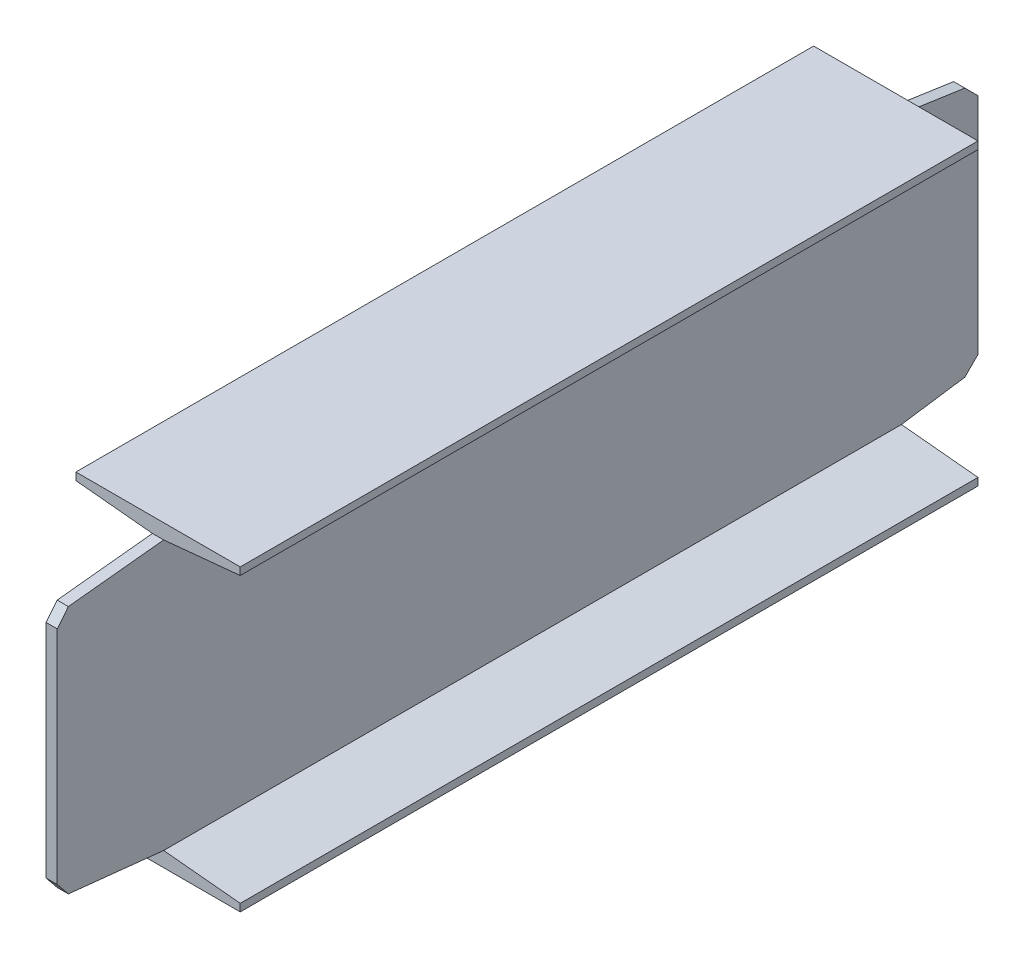
SolidWorks part; units mm, degrees
material "A3"
ref_plane "前视基准面" through (0, 0, 0) normal (0, 0, 1) x (1, 0, 0)
ref_plane "上视基准面" through (0, 0, 0) normal (0, 1, 0) x (1, 0, 0)
ref_plane "右视基准面" through (0, 0, 0) normal (1, 0, 0) x (0, 0, -1)
sketch "草图1" plane through (0, 0, 0) normal (0, 0, 1) x (1, 0, 0)
  line L0 (0, 80) -> (0, -80) construction
  line L1 (9.8926, 0) -> (-9.8926, 0) construction
  line L2 (44, 80) -> (-44, 80)
  line L3 (-44, 80) -> (-44, 76)
  line L4 (-44, 76) -> (-3, 72)
  line L5 (-3, 72) -> (-3, -72)
  line L6 (3, 72) -> (3, -72)
  line L7 (44, 76) -> (3, 72)
  line L8 (44, 80) -> (44, 76)
  line L9 (44, -80) -> (44, -76)
  line L10 (44, -76) -> (3, -72)
  line L11 (-44, -76) -> (-3, -72)
  line L12 (-44, -80) -> (-44, -76)
  line L13 (44, -80) -> (-44, -80)
  point P15 (0, 0)
  point P18 (3, 0)
  point P19 (-3, 0)
  dimension "D1" = 44
  dimension "D2" = 6
  dimension "D3" = 160
  dimension "D4" = 144
  dimension "D5" = 4
extrude "凸台-拉伸1" add sketch "草图1" along normal mid plane 493
sketch "草图3" plane through (0, 0, 0) normal (1, 0, 0) x (0, 0, -1)
  line L0 (-246.5, 66) -> (-189.5, 72)
  line L1 (-246.5, -72) -> (-246.5, 72) construction
  line L2 (-246.5, 72) -> (246.5, 72) construction
  line L3 (-189.5, 72) -> (-189.5, 80)
  line L4 (-246.5, 80) -> (246.5, 80) construction
  line L5 (-189.5, 80) -> (-246.5, 80)
  line L6 (-246.5, 80) -> (-246.5, 66)
  line L7 (0, 0) -> (0, 80) construction
  line L8 (246.5, 80) -> (246.5, 66)
  line L9 (205.5, 80) -> (246.5, 80)
  line L10 (205.5, 72) -> (205.5, 80)
  line L11 (246.5, 66) -> (205.5, 72)
  line L12 (0, 0) -> (246.5, 0) construction
  line L13 (246.5, -72) -> (246.5, 72) construction
  line L14 (246.5, -66) -> (205.5, -72)
  line L15 (205.5, -72) -> (205.5, -80)
  line L16 (205.5, -80) -> (246.5, -80)
  line L17 (246.5, -80) -> (246.5, -66)
  line L18 (-246.5, -80) -> (-246.5, -66)
  line L19 (-189.5, -80) -> (-246.5, -80)
  line L20 (-189.5, -72) -> (-189.5, -80)
  line L21 (-246.5, -66) -> (-189.5, -72)
  dimension "D1" = 57
  dimension "D2" = 66
  dimension "D3" = 41
extrude "切除-拉伸1" cut sketch "草图3" against normal through all both and the other way through all
chamfer "倒角1" distance 6 angle 45 4 edges at (0, -66, 246.5) (0, -66, -246.5) (0, 66, -246.5) (0, 66, 246.5)
